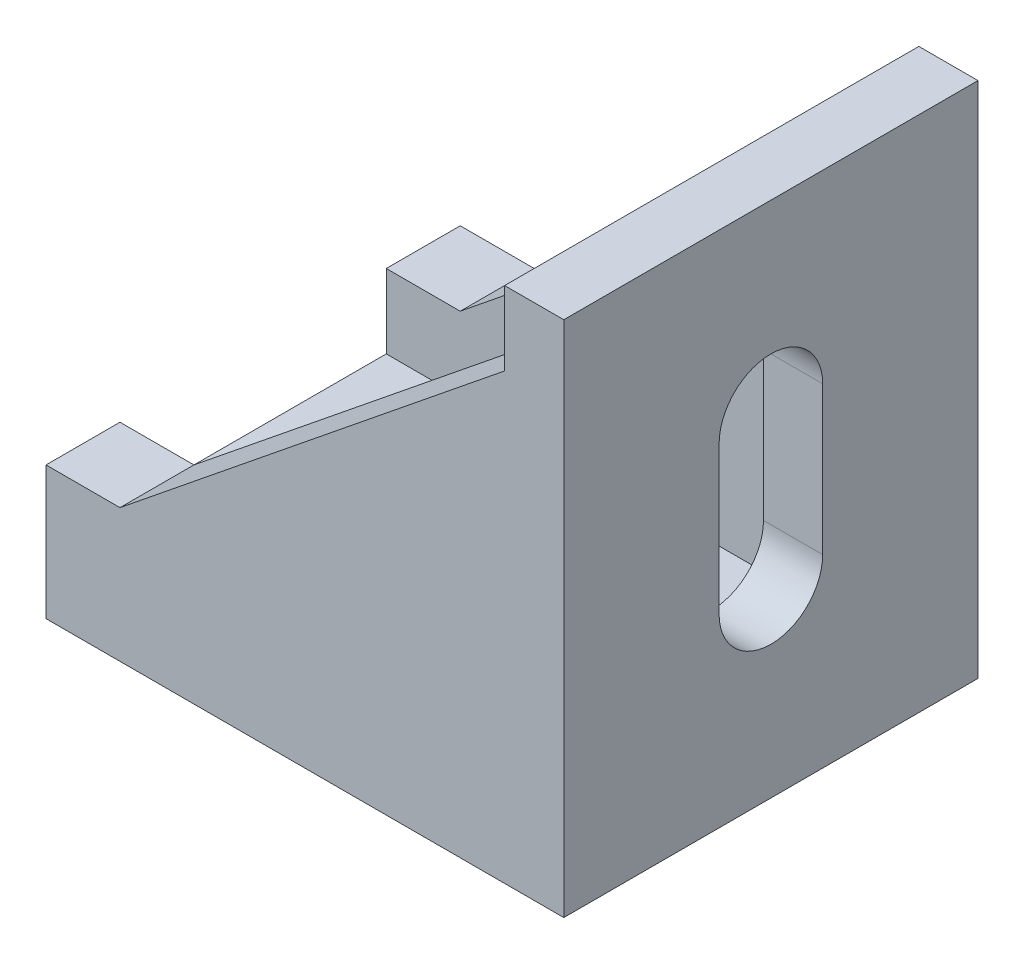
from build123d import *

# Parameters (mm, degrees)
SKETCH_1_W          = 4
SKETCH_1_H          = 31
SKETCH_1_H_2        = 4
SKETCH_1_W_2        = 31
EXTRUDE_1_DEPTH     = 14
EXTRUDE_2_DEPTH     = 5
CUT_EXTRUDE_1_DEPTH = 5
CUT_EXTRUDE_2_DEPTH = 5


with BuildPart() as part:
    # 草图1 → 凸台-拉伸1 (new, symmetric)
    with BuildSketch(Plane.XY):
        with Locations((0, 2)):
            Rectangle(SKETCH_1_W, SKETCH_1_H)
        with Locations((0, -15.5)):
            Rectangle(SKETCH_1_W, SKETCH_1_H_2)
        with Locations((-17.5, -15.5)):
            Rectangle(SKETCH_1_W_2, SKETCH_1_H_2)
    extrude(amount=EXTRUDE_1_DEPTH, both=True)

    # 草图2 → 凸台-拉伸2 (add)
    with BuildSketch(Plane(origin=(0, 0, -14), x_dir=(-1, 0, 0), z_dir=(0, 0, -1))):
        Polygon((2, 12.5), (28, -8.5), (33, -8.5), (33, -13.5), (2, -13.5), align=None)
    extrude_2 = extrude(amount=-EXTRUDE_2_DEPTH)

    # 镜向1: 凸台-拉伸2 across plane
    add(extrude_2.mirror(Plane.XY))

    # 草图3 → 切除-拉伸1 (cut)
    with BuildSketch(Plane.ZY.offset(2)):
        with BuildLine():
            Line((-3.5, -5), (-3.5, 5))
            ThreePointArc((-3.5, 5), (0, 8.5), (3.5, 5))
            Line((3.5, 5), (3.5, -5))
            ThreePointArc((3.5, -5), (0, -8.5), (-3.5, -5))
        make_face()
    extrude(amount=-CUT_EXTRUDE_1_DEPTH, mode=Mode.SUBTRACT)

    # 草图4 → 切除-拉伸2 (cut)
    with BuildSketch(Plane(origin=(0, -13.5, 0), x_dir=(1, 0, 0), z_dir=(0, 1, 0))):
        with BuildLine():
            Line((-20, 3.5), (-10, 3.5))
            ThreePointArc((-10, 3.5), (-6.5, 0), (-10, -3.5))
            Line((-10, -3.5), (-20, -3.5))
            ThreePointArc((-20, -3.5), (-23.5, 0), (-20, 3.5))
        make_face()
    extrude(amount=-CUT_EXTRUDE_2_DEPTH, mode=Mode.SUBTRACT)


solid = part.part
